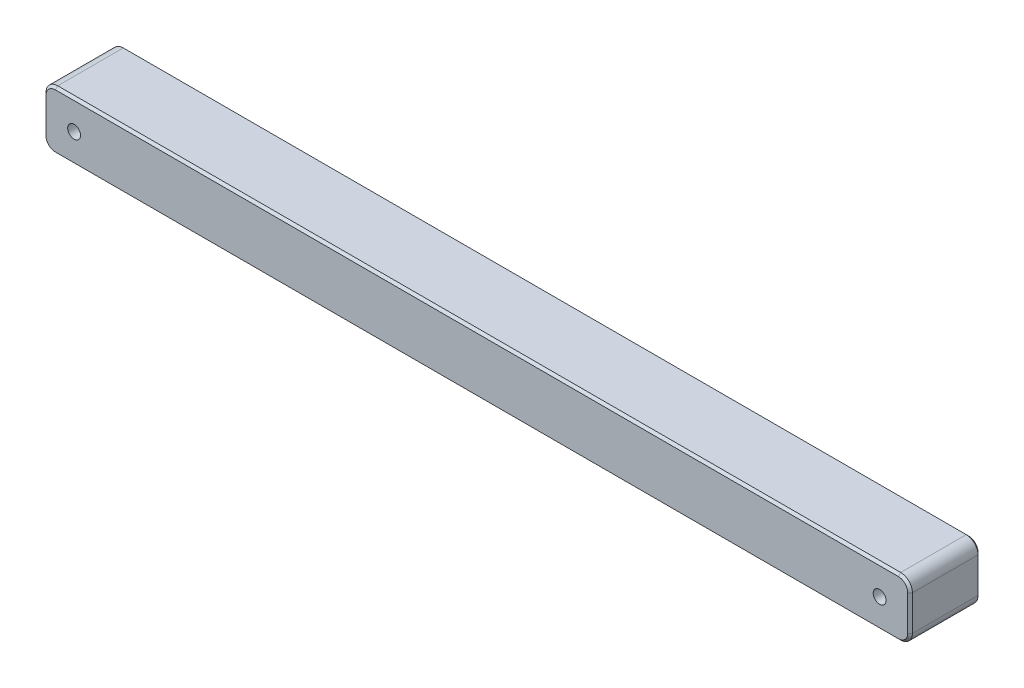
from build123d import *

# Parameters (mm, degrees)
SKETCH1_W                                            = 370
SKETCH1_H                                            = 25
BOSS_EXTRUDE1_DEPTH                                  = 15
FILLET1_R                                            = 5
CHAMFER1_SIZE                                        = 1
HOLE_SIZE_PER_SOCKET_HEAD_CAP_SCREW_TYPE_D           = 5.5
HOLE_SIZE_PER_SOCKET_HEAD_CAP_SCREW_TYPE_CBORE_D     = 10
HOLE_SIZE_PER_SOCKET_HEAD_CAP_SCREW_TYPE_CBORE_DEPTH = 5.7


with BuildPart() as part:
    # Sketch1 → Boss-Extrude1 (new, symmetric)
    with BuildSketch(Plane.XY):
        Rectangle(SKETCH1_W, SKETCH1_H)
    extrude(amount=BOSS_EXTRUDE1_DEPTH, both=True)

    # Fillet1
    fillet1_edges = [part.edges().sort_by_distance(p)[0] for p in [
        (185, -12.5, 0),
        (-185, -12.5, 0),
        (-185, 12.5, 0),
        (185, 12.5, 0),
    ]]
    fillet(fillet1_edges, radius=FILLET1_R)

    # Chamfer1
    chamfer1_edges = [part.edges().sort_by_distance(p)[0] for p in [
        (-185, 0, -15),
        (-185, 0, 15),
        (185, 0, -15),
        (0, -12.5, -15),
        (0, 12.5, -15),
        (183.535533906, 11.035533906, -15),
        (183.535533906, -11.035533906, -15),
        (-183.535533906, -11.035533906, -15),
        (-183.535533906, 11.035533906, -15),
        (0, 12.5, 15),
        (185, 0, 15),
        (0, -12.5, 15),
        (183.535533906, 11.035533906, 15),
        (183.535533906, -11.035533906, 15),
        (-183.535533906, -11.035533906, 15),
        (-183.535533906, 11.035533906, 15),
    ]]
    chamfer(chamfer1_edges, length=CHAMFER1_SIZE)

    # Hole size per socket head cap screw type 1 (through all)
    with Locations(Plane(origin=(0, 0, -15), x_dir=(-1, 0, 0), z_dir=(0, 0, -1))):
        with Locations((-172, 0), (172, 0)):
            CounterBoreHole(HOLE_SIZE_PER_SOCKET_HEAD_CAP_SCREW_TYPE_D / 2, HOLE_SIZE_PER_SOCKET_HEAD_CAP_SCREW_TYPE_CBORE_D / 2, HOLE_SIZE_PER_SOCKET_HEAD_CAP_SCREW_TYPE_CBORE_DEPTH)


solid = part.part
